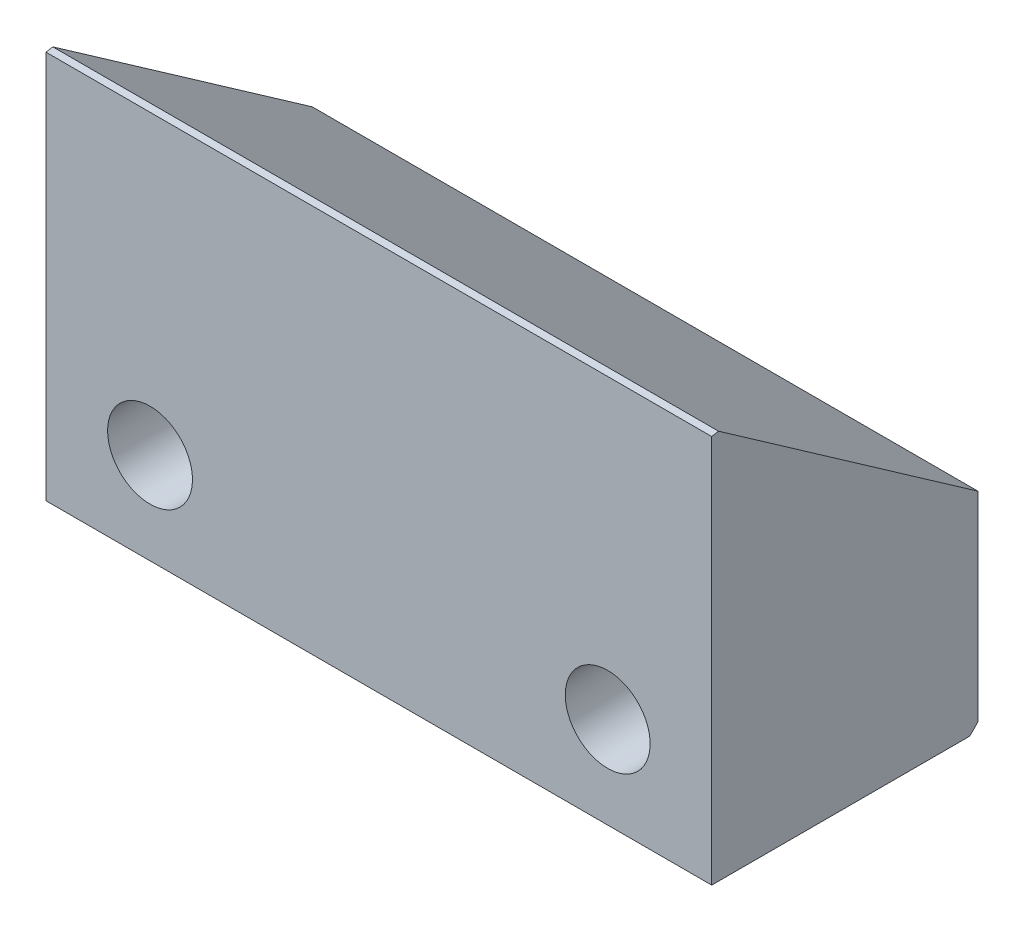
from build123d import *
from OCP.BRepFilletAPI import BRepFilletAPI_MakeChamfer

# Parameters (mm, degrees)
BOSS_EXTRUDE1_DEPTH = 80
CHAMFER1_SIZE       = 1
CHAMFER1_SIZE2      = 0.718015043


with BuildPart() as part:
    # Sketch1 → Boss-Extrude1 (new body)
    with BuildSketch(Plane(origin=(0, 0, 0), x_dir=(0, 0, -1), z_dir=(1, 0, 0))):
        Polygon((0, 0), (0, 47.406641223), (32, 25), (32, 0), align=None)
    extrude(amount=BOSS_EXTRUDE1_DEPTH)

    # Sketch3 → M12 Tapped Hole1 (revolve, cut)
    with BuildSketch(Plane(origin=(12.5, 11, -32), x_dir=(0, 1, 0), z_dir=(1, 0, 0))):
        Polygon((0, 0), (0, 63.064389157), (5.1, 60), (5.1, 0.925), (6.025, 0), align=None)
    m12_tapped_hole1 = revolve(axis=Axis((12.5, 11, -38.35), (0, 0, 1)), mode=Mode.SUBTRACT)

    # Mirror1: M12 Tapped Hole1 across plane
    add(m12_tapped_hole1.mirror(Plane(origin=(40, 0, 0), x_dir=(0, 0, 1), z_dir=(1, 0, 0))), mode=Mode.SUBTRACT)

    # Chamfer1: one chamfer whose edges measure the first distance from different faces: ONE call of the kernel's chamfer builder (chamfer() names one face for all edges)
    chamfer1_edges_1 = [part.edges().sort_by_distance(p)[0] for p in [
        (40, 47.406641223, 0),
    ]]
    chamfer1_side_1 = [part.faces().sort_by_distance(p)[0] for p in [
        (40, 36.203320611, -16),
    ]]
    chamfer1_edges_2 = [part.edges().sort_by_distance(p)[0] for p in [
        (40, 0, -32),
    ]]
    chamfer1 = BRepFilletAPI_MakeChamfer(part.part.solid().wrapped)
    for e in chamfer1_edges_1:
        chamfer1.Add(CHAMFER1_SIZE, CHAMFER1_SIZE2, e.wrapped, chamfer1_side_1[0].wrapped)  # the first distance lies on this face
    for e in chamfer1_edges_2:
        chamfer1.Add(CHAMFER1_SIZE, e.wrapped)
    add(Compound.cast(chamfer1.Shape()), mode=Mode.REPLACE)


solid = part.part
